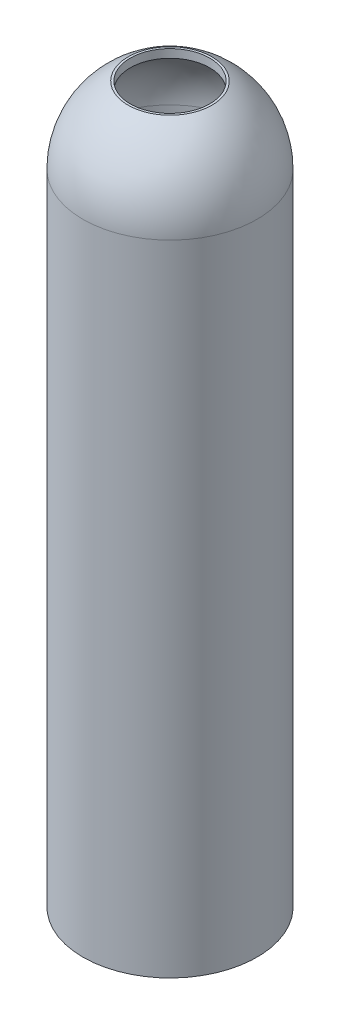
from build123d import *


with BuildPart() as part:
    # Sketch1 → Revolve1 (revolve)
    with BuildSketch(Plane.XY, mode=Mode.PRIVATE) as revolve1_sk:
        with BuildLine():
            Line((-2.18, 0), (-2.18, 16))
            ThreePointArc((-2.18, 16), (-1.876352845, 17.109819805), (-1.05, 17.910471146))
            Line((-1.05, 17.910471146), (-0.994634547, 17.910471146))
            Line((-0.994634547, 17.910471146), (-0.994634547, 17.700471146))
            ThreePointArc((-0.994634547, 17.700471146), (-1.708849036, 16.980170889), (-1.97, 16))
            Line((-1.97, 16), (-1.97, 0))
            Line((-1.97, 0), (-2.18, 0))
        make_face()
    revolve(revolve1_sk.sketch.rotate(Axis((0, 0, 0), (0, 1, 0)), 270), axis=Axis((0, 0, 0), (0, 1, 0)))


solid = part.part
